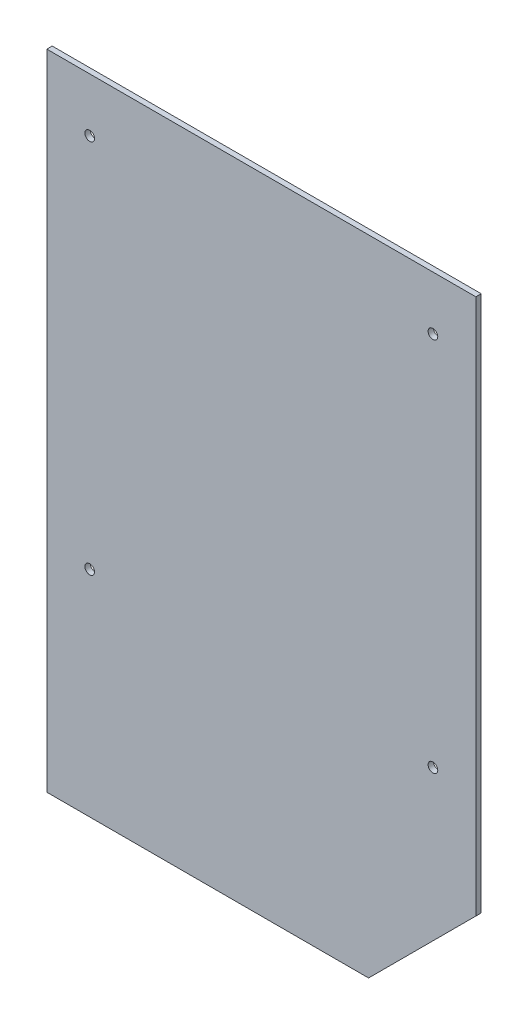
SolidWorks part; units mm, degrees
ref_plane "前视基准面" through (0, 0, 0) normal (0, 0, 1) x (1, 0, 0)
ref_plane "上视基准面" through (0, 0, 0) normal (0, 1, 0) x (1, 0, 0)
ref_plane "右视基准面" through (0, 0, 0) normal (1, 0, 0) x (0, 0, -1)
sketch "草图1" plane through (0, 0, 0) normal (0, 0, 1) x (1, 0, 0)
  line L1 (-200, -300) -> (200, -300)
  line L2 (-200, -300) -> (-200, 300)
  line L3 (-200, 300) -> (200, 300)
  line L4 (200, -300) -> (200, 300)
  line L5 (-200, -300) -> (200, 300) construction
  line L6 (-200, 300) -> (200, -300) construction
  point P0 (0, 0)
  dimension "D1" = 400
  dimension "D2" = 600
extrude "凸台-拉伸1" add sketch "草图1" along normal blind 5
sketch "草图2" plane through (0, 0, 5) normal (0, 0, 1) x (1, 0, 0)
  line L0 (0, 0) -> (0, 300) construction
  line L1 (200, 300) -> (-200, 300) construction
  circle A0 centre (-160, 250) radius 4.5
  circle A1 centre (160, 250) radius 4.5
  circle A2 centre (160, -100) radius 4.5
  circle A3 centre (-160, -100) radius 4.5
  dimension "D1" = 9
  dimension "D2" = 320
  dimension "D3" = 350
  dimension "D4" = 50
extrude "切除-拉伸1" cut sketch "草图2" against normal through all
chamfer "倒角1" distance 100 angle 45 1 edges at (200, -300, 2.5)
